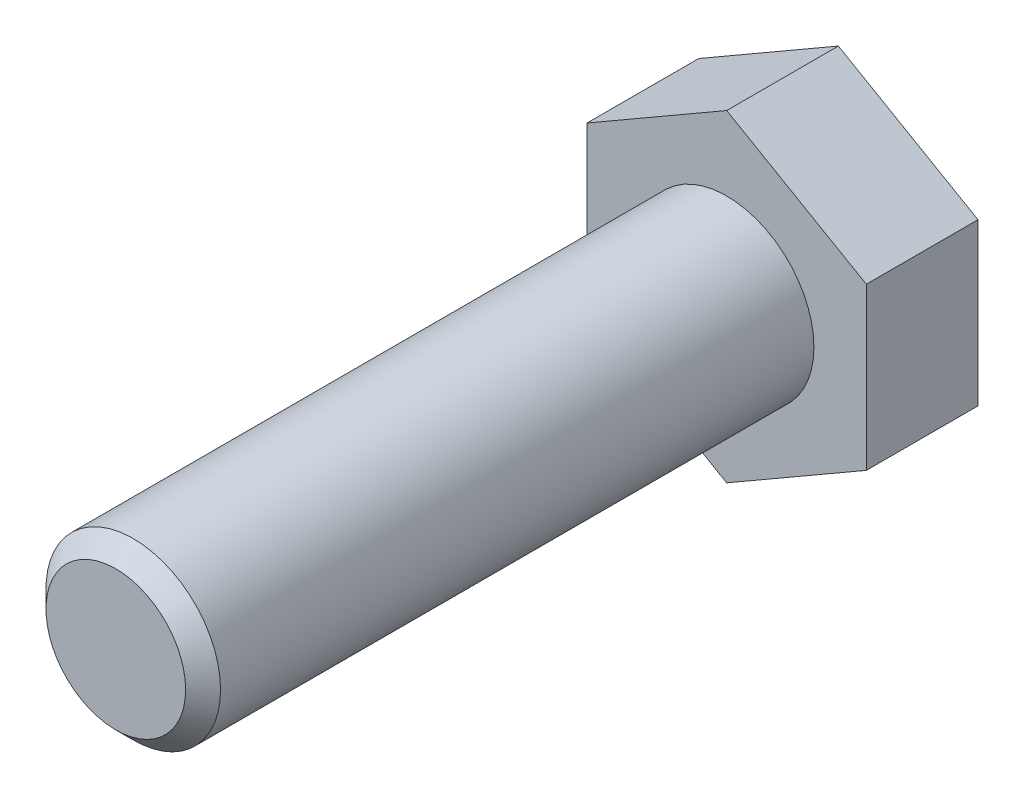
from build123d import *

# Parameters (mm, degrees)
BOSS_EXTRUDE1_DEPTH = 6.4
SKETCH3_R           = 5
BOSS_EXTRUDE2_DEPTH = 35
CHAMFER1_SIZE       = 1


with BuildPart() as part:
    # Sketch1 → Boss-Extrude1 (new body)
    with BuildSketch(Plane.XY):
        Polygon((8, 4.618802154), (0, 9.237604307), (-8, 4.618802154), (-8, -4.618802154), (0, -9.237604307), (8, -4.618802154), align=None)
    extrude(amount=BOSS_EXTRUDE1_DEPTH)

    # Sketch3 → Boss-Extrude2 (add)
    with BuildSketch(Plane.XY.offset(6.4)):
        Circle(SKETCH3_R)
    extrude(amount=BOSS_EXTRUDE2_DEPTH)

    # Chamfer1
    chamfer1_edges = [part.edges().sort_by_distance(p)[0] for p in [
        (-5, 0, 41.4),
    ]]
    chamfer(chamfer1_edges, length=CHAMFER1_SIZE)


solid = part.part
